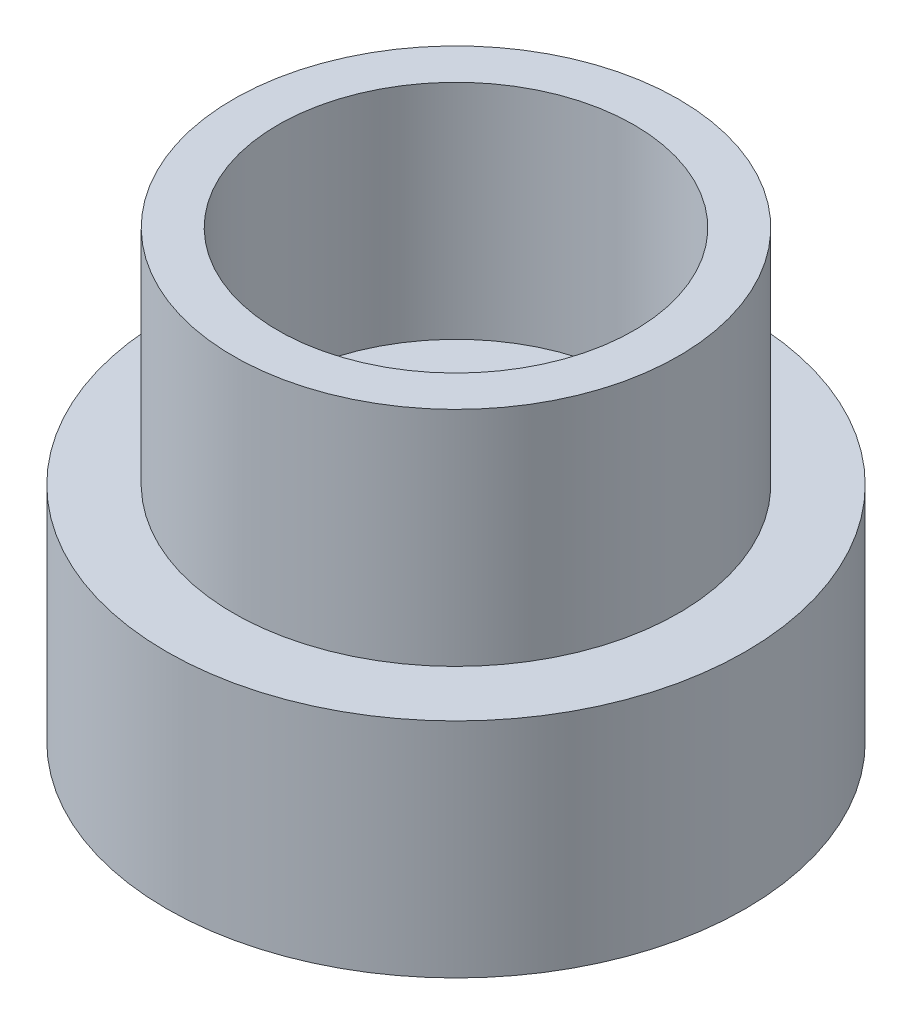
SolidWorks part; units mm, degrees
ref_plane "Front Plane" through (0, 0, 0) normal (0, 0, 1) x (1, 0, 0)
ref_plane "Top Plane" through (0, 0, 0) normal (0, 1, 0) x (1, 0, 0)
ref_plane "Right Plane" through (0, 0, 0) normal (1, 0, 0) x (0, 0, -1)
sketch "Sketch1" plane through (0, 0, 0) normal (0, 0, 1) x (1, 0, 0)
  line L0 (0, 0) -> (0, 10.9672) construction
  line L1 (0, 0) -> (6.5, 0)
  line L2 (6.5, 0) -> (6.5, 5)
  line L3 (6.5, 5) -> (5, 5)
  line L4 (5, 5) -> (5, 10)
  line L5 (5, 10) -> (4, 10)
  line L6 (4, 10) -> (4, 5)
  line L7 (4, 5) -> (0, 5)
  line L8 (0, 0) -> (0, 5)
  dimension "D1" = 5
  dimension "D2" = 1
  dimension "D3" = 5
  dimension "D4" = 6.5
  dimension "D5" = 10
revolve "Revolve1" add sketch "Sketch1" angle 360 about L0
